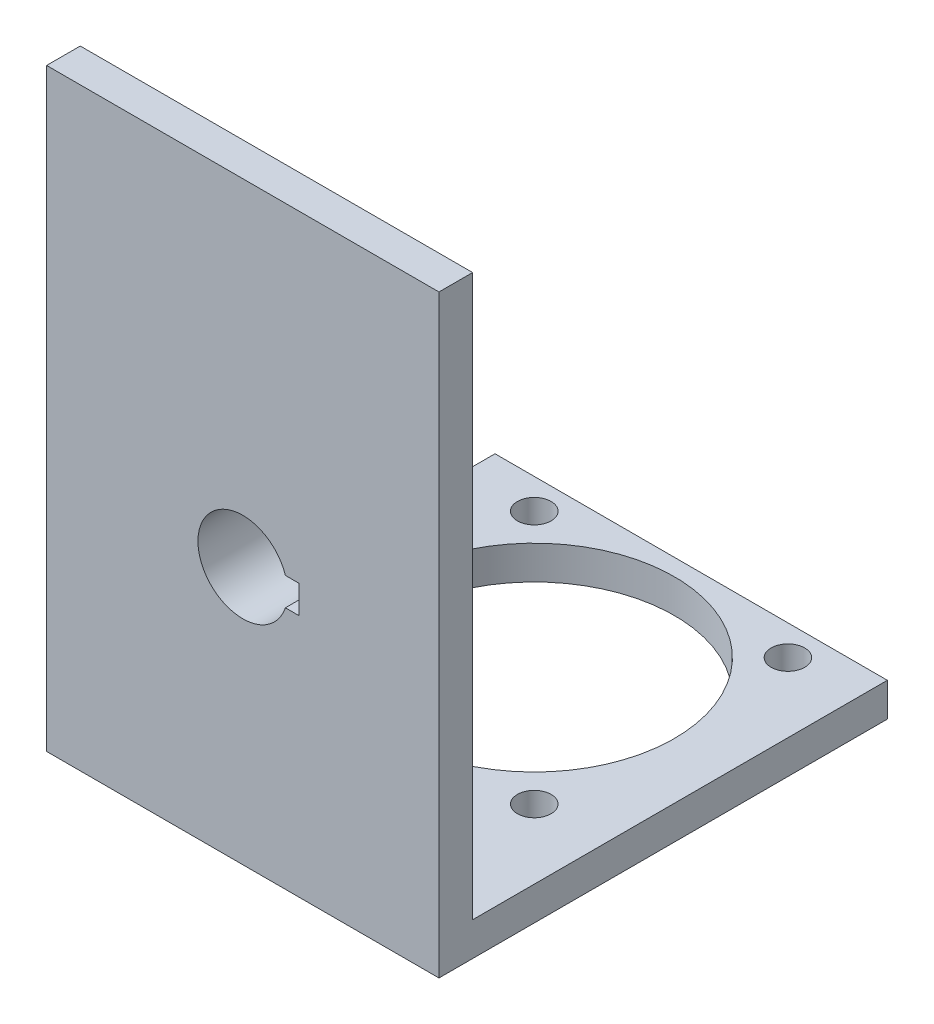
from build123d import *
from build123d.topology import SkipClean

# Parameters (mm, degrees)
SKETCH1_W           = 70
SKETCH1_H           = 100
SKETCH1_R           = 8
BOSS_EXTRUDE1_DEPTH = 6
BOSS_EXTRUDE2_START = 10
SKETCH2_R           = 18
SKETCH2_R_2         = 8
BOSS_EXTRUDE2_DEPTH = 10
SKETCH3_W           = 70
SKETCH3_H           = 80
BOSS_EXTRUDE3_DEPTH = 6
SKETCH4_W           = 4.928950204
SKETCH4_H           = 5
CUT_EXTRUDE1_DEPTH  = 95.451045521
SKETCH5_R           = 3.006498603
SKETCH5_R_2         = 3
SKETCH5_R_3         = 25.009138209
CUT_EXTRUDE2_DEPTH  = 6


with BuildPart() as part:
    # Sketch1 → Boss-Extrude1 (new body)
    with BuildSketch(Plane.XY):
        with Locations((0, 10)):
            Rectangle(SKETCH1_W, SKETCH1_H)
        Circle(SKETCH1_R, mode=Mode.SUBTRACT)
    extrude(amount=BOSS_EXTRUDE1_DEPTH)

    # Sketch2 → Boss-Extrude2 (add)
    with SkipClean():  # the faces are left unmerged after this step: merging them gives an invalid solid
        with BuildSketch(Plane(origin=(0, 0, 0), x_dir=(-1, 0, 0), z_dir=(0, 0, -1)).offset(BOSS_EXTRUDE2_START)):
            with Locations(Location((0, 0, 0), (0, 0, 180))):
                Circle(SKETCH2_R)
            Circle(SKETCH2_R_2, mode=Mode.SUBTRACT)
        extrude(amount=-BOSS_EXTRUDE2_DEPTH)

    # Sketch3 → Boss-Extrude3 (add)
    with SkipClean():  # the faces are left unmerged after this step: merging them gives an invalid solid
        with BuildSketch(Plane.XZ.offset(40)):
            with Locations((0, -34)):
                Rectangle(SKETCH3_W, SKETCH3_H)
        extrude(amount=BOSS_EXTRUDE3_DEPTH)

    # Sketch4 → Cut-Extrude1 (cut, through all)
    with BuildSketch(Plane(origin=(0, 0, -10), x_dir=(-1, 0, 0), z_dir=(0, 0, -1))):
        with Locations((-7.535524898, 0)):
            Rectangle(SKETCH4_W, SKETCH4_H)
    extrude(amount=-CUT_EXTRUDE1_DEPTH, mode=Mode.SUBTRACT)

    # Sketch5 → Cut-Extrude2 (cut)
    with BuildSketch(Plane(origin=(0, -40, 0), x_dir=(1, 0, 0), z_dir=(0, 1, 0))):
        with Locations(Location((-22.627416998, 68.627416998, 0), (0, 0, 270))):
            Circle(SKETCH5_R)
        with Locations(Location((22.627416998, 68.627416998, 0), (0, 0, 270))):
            Circle(SKETCH5_R_2)
        with Locations(Location((22.627416998, 23.372583002, 0), (0, 0, 270))):
            Circle(SKETCH5_R_2)
        with Locations(Location((-22.627416998, 23.372583002, 0), (0, 0, 270))):
            Circle(SKETCH5_R_2)
        with Locations(Location((-0.009138209, 46.00000012, 0), (0, 0, 270))):
            Circle(SKETCH5_R_3)
    extrude(amount=-CUT_EXTRUDE2_DEPTH, mode=Mode.SUBTRACT)


solid = part.part
